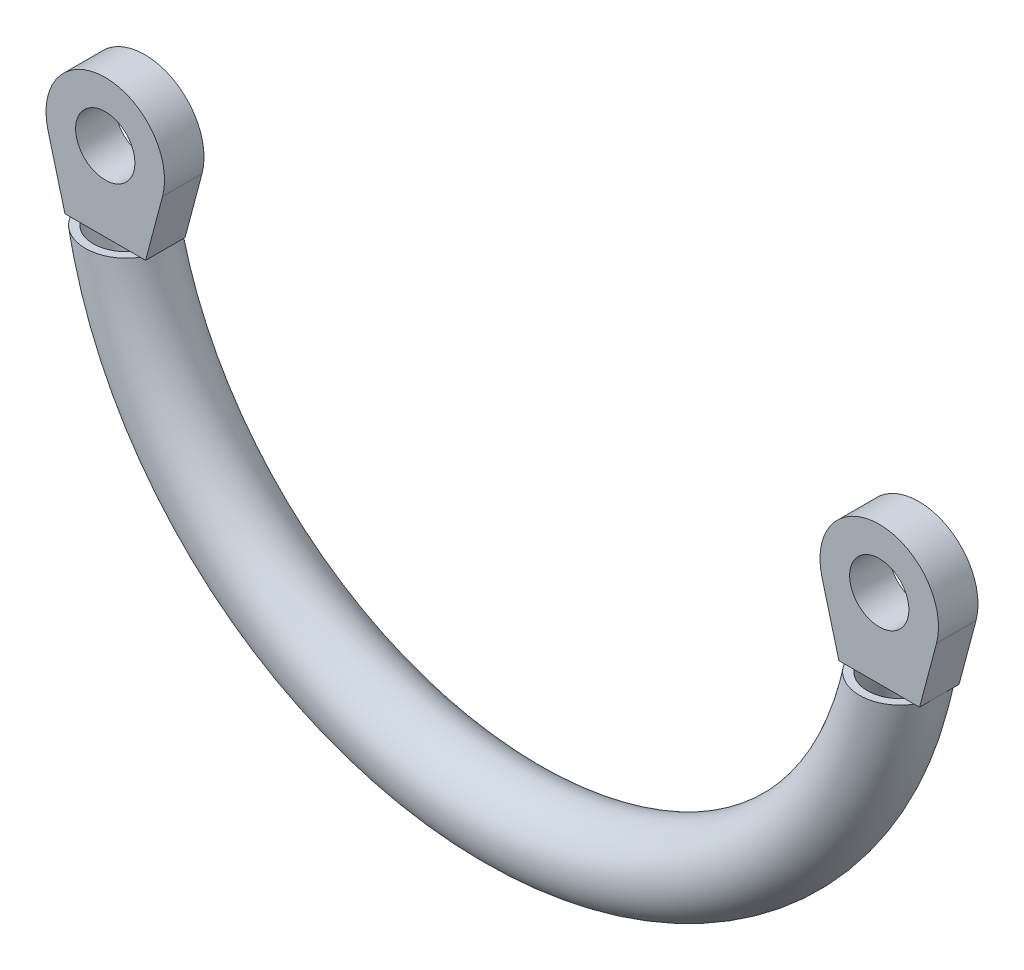
from build123d import *

# Parameters (mm, degrees)
SKETCH_2_R               = 10
SKETCH_2_R_2             = 8
CUT_EXTRUDE_1_DEPTH      = 156.884572829
CUT_EXTRUDE_1_DEPTH_BACK = 156.884572829
SKETCH_4_R               = 7.5
EXTRUDE_1_DEPTH          = 5


with BuildPart() as part:
    # 扫描1: sweep along a path in 草图1
    with BuildLine(Plane.XY) as sweep_1_path:
        CenterArc((0, 0), 100, 0, 360)
    # 草图2 → 扫描1 (sweep)
    with BuildSketch(Plane(origin=(0, 0, 0), x_dir=(0, 0, -1), z_dir=(1, 0, 0))):
        with Locations((0, -100)):
            Circle(SKETCH_2_R)
        with Locations((0, -100)):
            Circle(SKETCH_2_R_2, mode=Mode.SUBTRACT)
    sweep(path=sweep_1_path.line)

    # 草图3 → 切除-拉伸1 (cut, two sides: drawn at the far end of the back side and taken through both)
    with BuildSketch(Plane.XY.offset(-CUT_EXTRUDE_1_DEPTH_BACK)):
        Polygon((-124.821104754, -20), (0, -20), (127.823184446, -20), (127.823184446, 142.660997567), (-124.821104754, 142.660997567), align=None)
    extrude(amount=CUT_EXTRUDE_1_DEPTH + CUT_EXTRUDE_1_DEPTH_BACK, mode=Mode.SUBTRACT)

    # 草图4 → 凸台-拉伸1 (add, symmetric)
    with BuildSketch(Plane.XY):
        with BuildLine():
            Line((-108.166537158, -20.000005979), (-112.455542967, -3.850181648))
            ThreePointArc((-112.455542967, -3.850181648), (-97.958089835, 14.999994021), (-83.460636703, -3.850181648))
            Line((-83.460636703, -3.850181648), (-87.749642511, -20.000005979))
            Line((-87.749642511, -20.000005979), (-108.166537158, -20.000005979))
        make_face()
        with Locations((-97.958089835, -5.979e-06)):
            Circle(SKETCH_4_R, mode=Mode.SUBTRACT)
    extrude_1 = extrude(amount=EXTRUDE_1_DEPTH, both=True)

    # 镜向1: 凸台-拉伸1 across plane
    add(extrude_1.mirror(Plane(origin=(0, 0, 0), x_dir=(0, 0, 1), z_dir=(1, 0, 0))))


solid = part.part
